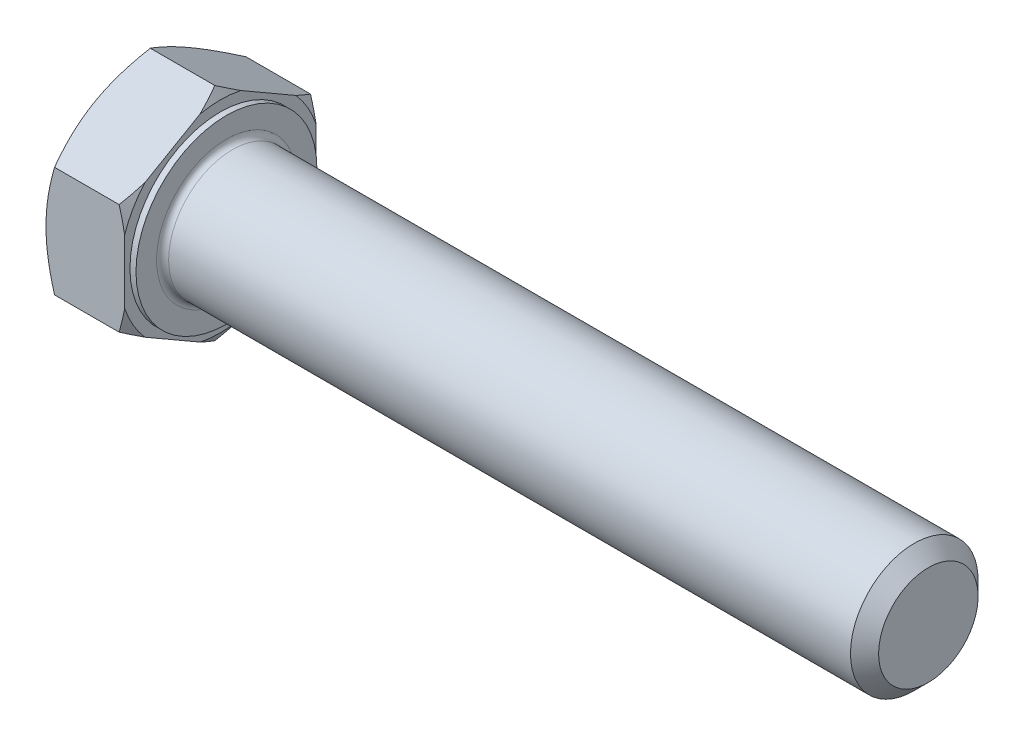
SolidWorks part; units mm, degrees
material "SAE2"
ref_plane "Front Plane" through (0, 0, 0) normal (0, 0, 1) x (1, 0, 0)
ref_plane "Top Plane" through (0, 0, 0) normal (0, 1, 0) x (1, 0, 0)
ref_plane "Right Plane" through (0, 0, 0) normal (1, 0, 0) x (0, 0, -1)
sketch "Sketch1" plane through (0, 0, 0) normal (1, 0, 0) x (0, 0, -1)
  line L0 (9.525, 5.4993) -> (9.525, -5.4993)
  line L1 (-9.525, 5.4993) -> (-9.525, -5.4993)
  line L2 (9.525, -5.4993) -> (0, -10.9985)
  line L3 (0, -10.9985) -> (-9.525, -5.4993)
  line L4 (9.525, 5.4993) -> (0, 10.9985)
  line L5 (0, 10.9985) -> (-9.525, 5.4993)
  dimension "s" = 19.05
  dimension "D2" = 120
  dimension "D3" = 9.525
  dimension "D4" = 9.525
  dimension "D5" = 9.525
extrude "Base-Extrude" add sketch "Sketch1" along normal blind 8.7312
sketch "Sketch2" plane through (0, 0, 0) normal (0, 0, 1) x (1, 0, 0)
  line L0 (0, 5.4993) -> (0, -5.4993) construction
  line L1 (0, 0) -> (78.5812, 0)
  line L2 (0, 0) -> (0, 6.35)
  line L3 (0, 6.35) -> (27.8072, 6.35)
  line L4 (78.5812, 0) -> (78.5812, 5.5562)
  line L5 (8.7312, 10.9985) -> (8.7312, 5.4993) construction
  line L7 (0, 0) -> (96.52, 0) construction
  line L8 (78.5812, -5.5562) -> (27.8072, -6.35) construction
  line L9 (0, -6.35) -> (27.8072, -6.35) construction
  line L10 (10.4812, 15.24) -> (10.4813, -1.27) construction
  line L11 (46.8312, 15.24) -> (46.8312, -1.27) construction
  line L12 (8.7312, 5.4993) -> (8.7312, -5.4993) construction
  line L13 (27.8072, 6.35) -> (78.5812, 6.35)
  line L14 (78.5812, 6.35) -> (78.5812, 5.5562)
  dimension "l" = 69.85
  dimension "m" = 12.7
  dimension "Minor_dia" = 11.1125
  dimension "p" = 1.75
  dimension "h" = 31.75
revolve "Boss-Revolve1" add sketch "Sketch2" angle 360 about L7
cosmetic thread "Helix1" parameters "Thread_length"=30, "Thread_minor"=8.969
sketch "Sketch3" plane through (0, 0, 0) normal (0, 0, 1) x (1, 0, 0)
  line L0 (0, 9) -> (4.0406, 15.9985)
  line L1 (0, 10.9985) -> (0, 5.4993) construction
  line L2 (4.0406, 15.9985) -> (4.0406, 20.9985)
  line L3 (4.0406, 20.9985) -> (-10, 20.9985)
  line L4 (-10, 20.9985) -> (-10, 9)
  line L5 (-10, 9) -> (0, 9)
  line L6 (0, 0) -> (99.06, 0) construction
  line L7 (8.7312, 10.9985) -> (0, 10.9985) construction
  dimension "D1" = 9
  dimension "D2" = 5
  dimension "D3" = 10
  dimension "D4" = 5
  dimension "Head_ch_ang" = 30
revolve "Cut-Revolve1" cut sketch "Sketch3" angle 360 about L6
sketch "Sketch5" plane through (0, 0, 0) normal (0, 0, 1) x (1, 0, 0)
  line L0 (8.7312, 9) -> (4.6907, 15.9985)
  line L1 (8.7312, 10.9985) -> (8.7312, 5.4993) construction
  line L2 (4.6907, 15.9985) -> (4.6907, 20.9985)
  line L3 (4.6907, 20.9985) -> (14.6907, 20.9985)
  line L4 (14.6907, 20.9985) -> (14.6907, 9)
  line L5 (14.6907, 9) -> (8.7312, 9)
  line L7 (8.7312, 10.9985) -> (1.1538, 10.9985) construction
  line L8 (0, 0) -> (99.06, 0) construction
  line L9 (0, 0) -> (99.06, 0) construction
  dimension "D1" = 9
  dimension "D2" = 5
  dimension "D3" = 10
  dimension "Head_ch_ang" = 30
  dimension "D4" = 5
revolve "Cut-Revolve2" cut sketch "Sketch5" angle 360 about L8
sketch "Sketch4" plane through (0, 0, 0) normal (0, 0, 1) x (1, 0, 0)
  line L1 (8.7312, 10.9985) -> (8.7312, 5.4993) construction
  line L2 (8.7312, 9) -> (8.1312, 9)
  line L3 (8.7312, 9) -> (8.7312, 20.9985)
  line L4 (8.7312, 20.9985) -> (8.1312, 20.9985)
  line L5 (0, 0) -> (95.25, 0) construction
  line L6 (0, 0) -> (96.52, 0) construction
  line L7 (8.1312, 9) -> (8.1312, 20.9985)
  line L8 (7.5774, 10.9985) -> (1.1538, 10.9985) construction
  dimension "D1" = 18
  dimension "D2" = 10
  dimension "c" = 0.6
revolve "Cut-Revolve3" cut sketch "Sketch4" angle 360 about L5
chamfer "Chamfer" distance 1.4 angle 45 1 edges at (78.5812, 0, 6.35)
fillet "Fillet" radius 0.6 1 edges at (8.7312, 0, -6.35)
sketch "Sketch6" plane through (0, 0, 0) normal (0, 0, 1) x (1, 0, 0)
  line L0 (77.5, -4.4845) -> (76.625, -6)
  line L1 (77.5, -4.4845) -> (78.375, -6)
  line L2 (78.375, -6) -> (78.375, -7.5)
  line L3 (-3.175, 0) -> (5.1513, 0) construction
  line L5 (78.375, -7.5) -> (76.625, -7.5)
  line L6 (76.625, -7.5) -> (76.625, -6)
  dimension "Thread_minor" = 8.969
  dimension "Diameter" = 12
  dimension "Start" = 77.5
  dimension "SideAngle" = 60
  dimension "VeeAngle" = 60
  dimension "Overcut" = 15
revolve "Cut-Revolve4" [suppressed] cut sketch "Sketch6" angle 360 about L3
pattern_linear "LPattern1" [suppressed]
